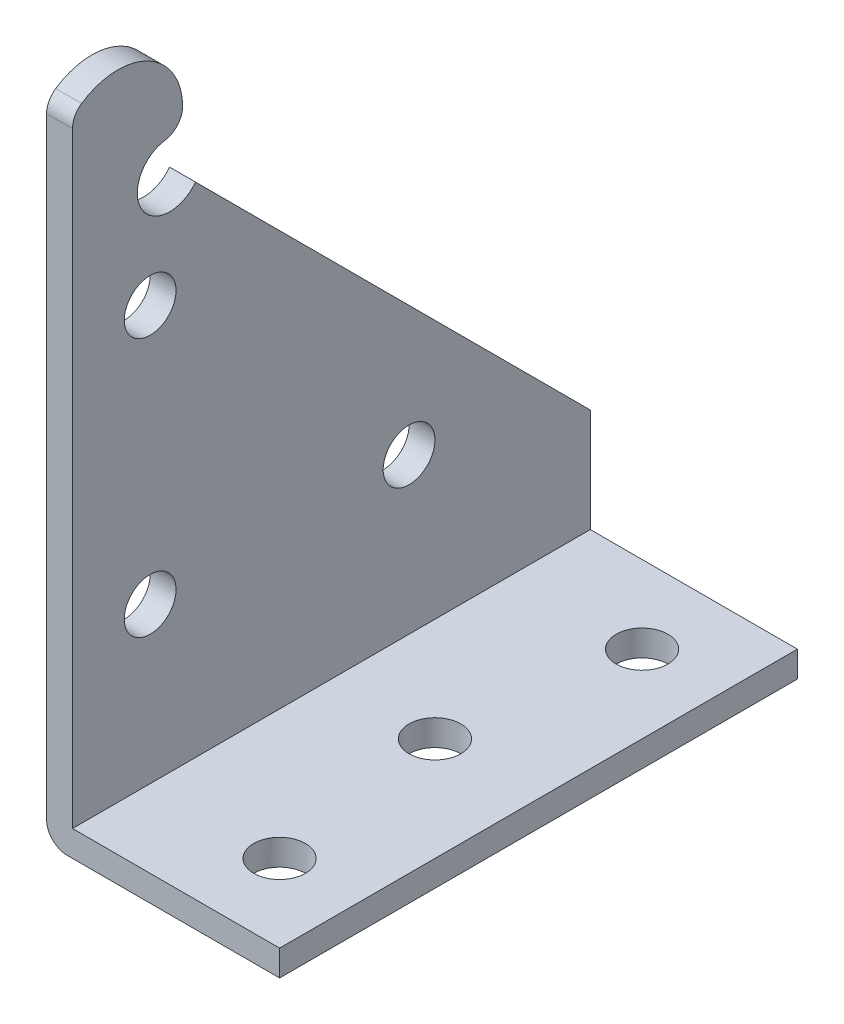
SolidWorks part; units mm, degrees
ref_plane "Front Plane" through (0, 0, 0) normal (0, 0, 1) x (1, 0, 0)
ref_plane "Top Plane" through (0, 0, 0) normal (0, 1, 0) x (1, 0, 0)
ref_plane "Right Plane" through (0, 0, 0) normal (1, 0, 0) x (0, 0, -1)
sketch "Sketch1" plane through (0, 0, 0) normal (1, 0, 0) x (0, 0, -1)
  line L0 (0, 0) -> (63.5, 0)
  line L1 (63.5, 0) -> (63.5, 15.875)
  line L2 (63.5, 15.875) -> (15.0803, 64.2947)
  line L3 (0, 77.5121) -> (0, 0)
  line L4 (0, 3.175) -> (63.5, 3.175)
  circle A0 centre (9.525, 53.975) radius 3.175
  circle A1 centre (9.525, 22.225) radius 3.175
  circle A2 centre (41.275, 22.225) radius 3.175
  arc A4 (15.0803, 64.2947) -> (11.3395, 70.5957) centre (11.9126, 66.675) cw
  arc A5 (1.1209, 79.6187) -> (13.5118, 73.1485) centre (5.5626, 73.025) cw
  arc A6 (13.5118, 73.1485) -> (11.3395, 70.5957) centre (10.9721, 73.109) cw
  arc A7 (0, 77.5121) -> (1.1209, 79.6187) centre (2.54, 77.5121) cw
  point P11 (5.5626, 73.025)
  point P15 (11.9126, 66.675)
  dimension "D4" = 6.35
  dimension "D5" = 6.35
  dimension "D6" = 6.35
  dimension "D13" = 7.9502
  dimension "D16" = 3.9624
  dimension "D17" = 2.54
  dimension "D1" = 63.5
  dimension "D2" = 15.875
  dimension "D3" = 45
  dimension "D7" = 9.525
  dimension "D8" = 31.75
  dimension "D9" = 22.225
  dimension "D10" = 31.75
  dimension "D11" = 19.05
  dimension "D12" = 5.5626
  dimension "D14" = 6.35
  dimension "D15" = 6.35
  dimension "D18" = 3.175
extrude "Boss-Extrude1" add sketch "Sketch1" against normal blind 3.175 contours A7 L3 L4 L1 L2 A4 A6 A5 A2 A1 A0 | L4 L3 L0 L1
sketch "Sketch2" plane through (0, 0, 0) normal (1, 0, 0) x (0, 0, -1)
  line L0 (63.5, 0) -> (63.5, 15.875) construction
  line L1 (0, 0) -> (63.5, 0)
  line L2 (0, 0) -> (0, 3.175)
  line L3 (0, 3.175) -> (63.5, 3.175)
  line L4 (63.5, 0) -> (63.5, 3.175)
  dimension "D1" = 3.175
extrude "Boss-Extrude2" add sketch "Sketch2" along normal blind 25.4
sketch "Sketch3" plane through (0, 0, 0) normal (0, 0, 1) x (1, 0, 0)
  line L0 (-3.175, 4.7442) -> (-3.175, 2.54)
  line L1 (-3.175, 77.5121) -> (-3.175, 0) construction
  line L2 (-0.635, 0) -> (1.0329, 0)
  line L3 (-3.175, 0) -> (25.4, 0) construction
  line L4 (-3.175, 2.54) -> (-3.175, 0)
  line L5 (-3.175, 0) -> (-0.635, 0)
  arc A0 (-0.635, 0) -> (-3.175, 2.54) centre (-0.635, 2.54) cw
  point P10 (-3.175, 0)
  line M3 (-3.175, 77.5121) -> (-3.175, 0)
  line M4 (-3.175, 0) -> (25.4, 0)
  dimension "D1" = 2.54
extrude "Cut-Extrude1" cut sketch "Sketch3" against normal through all contours A0 M4 M3
sketch "Sketch4" plane through (0, 3.175, 0) normal (0, 1, 0) x (1, 0, 0)
  line L0 (25.4, 63.5) -> (25.4, 0) construction
  line L1 (25.4, 0) -> (0, 0) construction
  line L2 (25.4, 63.5) -> (0, 63.5) construction
  circle A0 centre (15.875, 53.975) radius 3.175
  circle A1 centre (12.7, 31.75) radius 3.175
  circle A2 centre (15.875, 9.525) radius 3.175
  point P10 (0, 0)
  dimension "D1" = 6.35
  dimension "D2" = 6.35
  dimension "D3" = 6.35
  dimension "D4" = 9.525
  dimension "D5" = 9.525
  dimension "D6" = 9.525
  dimension "D7" = 31.75
  dimension "D8" = 3.175
extrude "Cut-Extrude2" cut sketch "Sketch4" against normal blind 25.4 contours A0 | A1 | A2
